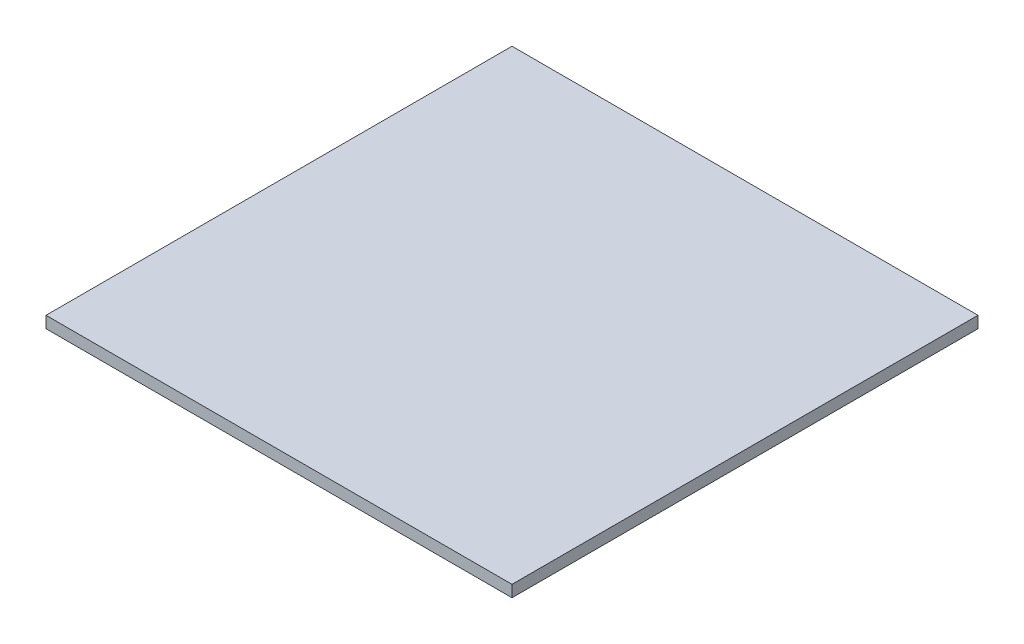
from build123d import *

# Parameters (mm, degrees)
SKETCH1_W           = 80
SKETCH1_H           = 80
BOSS_EXTRUDE1_DEPTH = 2


with BuildPart() as part:
    # Sketch1 → Boss-Extrude1 (new body)
    with BuildSketch(Plane(origin=(0, 0, 0), x_dir=(1, 0, 0), z_dir=(0, 1, 0))):
        Rectangle(SKETCH1_W, SKETCH1_H)
    extrude(amount=BOSS_EXTRUDE1_DEPTH)


solid = part.part
